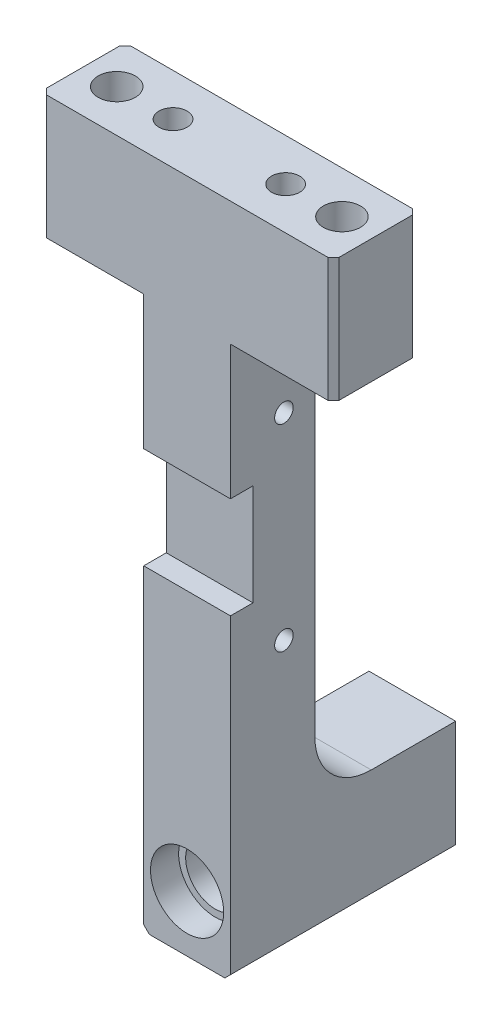
from build123d import *

# Parameters (mm, degrees)
SKETCH1_W                     = 52
SKETCH1_H                     = 120
BOSS_EXTRUDE1_DEPTH           = 7.5
SKETCH8_W                     = 18.3
SKETCH8_H                     = 98
CUT_EXTRUDE4_DEPTH            = 68.089492471
F_6_6_6_6_DIAMETER_HOLE1_D    = 6.6
CHAMFER1_SIZE                 = 1
BLIND_PIN_HOLE1_SIZE_MM_D     = 5
BLIND_PIN_HOLE1_SIZE_MM_DEPTH = 11
BLIND_PIN_HOLE1_SIZE_MM_TIP   = 1.502151548
BOSS_EXTRUDE2_DEPTH           = 25
FILLET1_R                     = 10
SKETCH14_R                    = 5.25
CUT_EXTRUDE5_DEPTH            = 77.655071587
SKETCH15_R                    = 6.5
CUT_EXTRUDE6_DEPTH            = 5
CUT_EXTRUDE7_START            = -5
SKETCH16_R                    = 6.5
CUT_EXTRUDE7_DEPTH            = 5
SKETCH17_W                    = 4
SKETCH17_H                    = 18
CUT_EXTRUDE8_DEPTH            = 77.104796169
M4_TAPPED_HOLE1_D             = 3.3
M4_TAPPED_HOLE1_DEPTH         = 10.1
M4_TAPPED_HOLE1_TIP           = 0.991420021


with BuildPart() as part:
    # Sketch1 → Boss-Extrude1 (new, symmetric)
    with BuildSketch(Plane.XY):
        Rectangle(SKETCH1_W, SKETCH1_H)
    extrude(amount=BOSS_EXTRUDE1_DEPTH, both=True)

    # Sketch8 → Cut-Extrude4 (cut, through all)
    with BuildSketch(Plane.XY.offset(7.5)):
        with Locations((-16.85, -11)):
            Rectangle(SKETCH8_W, SKETCH8_H)
    cut_extrude4 = extrude(amount=-CUT_EXTRUDE4_DEPTH, mode=Mode.SUBTRACT)

    # Mirror1: Cut-Extrude4 across plane
    add(cut_extrude4.mirror(Plane(origin=(0, 0, 0), x_dir=(0, 0, 1), z_dir=(1, 0, 0))), mode=Mode.SUBTRACT)

    # Ø6.6 (6.6) Diameter Hole1 (through all)
    with Locations(Plane(origin=(0, 60, 0), x_dir=(1, 0, 0), z_dir=(0, 1, 0))):
        with Locations((-20, 0), (20, 0)):
            Hole(F_6_6_6_6_DIAMETER_HOLE1_D / 2)

    # Chamfer1
    chamfer1_edges = [part.edges().sort_by_distance(p)[0] for p in [
        (-26, 49, 7.5),
        (-7.7, -60, 0),
        (26, 49, -7.5),
        (26, 49, 7.5),
        (7.7, -60, 0),
        (-26, 49, -7.5),
    ]]
    chamfer(chamfer1_edges, length=CHAMFER1_SIZE)

    # Blind Pin Hole1 size mm
    with Locations(Plane(origin=(0, 60, 0), x_dir=(1, 0, 0), z_dir=(0, 1, 0))):
        with Locations((-10, 0), (10, 0)):
            Hole(BLIND_PIN_HOLE1_SIZE_MM_D / 2, depth=BLIND_PIN_HOLE1_SIZE_MM_DEPTH)
            with Locations((0, 0, -(BLIND_PIN_HOLE1_SIZE_MM_DEPTH + BLIND_PIN_HOLE1_SIZE_MM_TIP / 2))):  # 118° drill point
                Cone(0, BLIND_PIN_HOLE1_SIZE_MM_D / 2, BLIND_PIN_HOLE1_SIZE_MM_TIP, mode=Mode.SUBTRACT)

    # Sketch13 → Boss-Extrude2 (add)
    with BuildSketch(Plane(origin=(0, 0, -7.5), x_dir=(-1, 0, 0), z_dir=(0, 0, -1))):
        Polygon((-7.7, -40), (7.7, -40), (7.7, -59), (6.7, -60), (-6.7, -60), (-7.7, -59), align=None)
    extrude(amount=BOSS_EXTRUDE2_DEPTH)

    # Fillet1
    fillet1_edges = [part.edges().sort_by_distance(p)[0] for p in [
        (0, -40, -7.5),
    ]]
    fillet(fillet1_edges, radius=FILLET1_R)

    # Sketch14 → Cut-Extrude5 (cut, through all)
    with BuildSketch(Plane.XY.offset(7.5)):
        with Locations((0, -50)):
            Circle(SKETCH14_R)
    extrude(amount=-CUT_EXTRUDE5_DEPTH, mode=Mode.SUBTRACT)

    # Sketch15 → Cut-Extrude6 (cut)
    with BuildSketch(Plane.XY.offset(7.5)):
        with Locations((0, -50)):
            Circle(SKETCH15_R)
    extrude(amount=-CUT_EXTRUDE6_DEPTH, mode=Mode.SUBTRACT)

    # Sketch16 → Cut-Extrude7 (cut)
    with BuildSketch(Plane(origin=(0, 0, -32.5), x_dir=(-1, 0, 0), z_dir=(0, 0, -1)).offset(CUT_EXTRUDE7_START)):
        with Locations(Location((0, -50, 0), (0, 0, 180))):
            Circle(SKETCH16_R)
    extrude(amount=CUT_EXTRUDE7_DEPTH, mode=Mode.SUBTRACT)

    # Sketch17 → Cut-Extrude8 (cut, through all)
    with BuildSketch(Plane(origin=(7.7, 0, 0), x_dir=(0, 0, -1), z_dir=(1, 0, 0))):
        with Locations((-5.5, 5.2)):
            Rectangle(SKETCH17_W, SKETCH17_H)
    extrude(amount=-CUT_EXTRUDE8_DEPTH, mode=Mode.SUBTRACT)

    # M4 Tapped Hole1
    with Locations(Plane(origin=(7.7, 0, 0), x_dir=(0, 0, -1), z_dir=(1, 0, 0))):
        with Locations((2, 22.7), (2, -12.3)):
            Hole(M4_TAPPED_HOLE1_D / 2, depth=M4_TAPPED_HOLE1_DEPTH)
            with Locations((0, 0, -(M4_TAPPED_HOLE1_DEPTH + M4_TAPPED_HOLE1_TIP / 2))):  # 118° drill point
                Cone(0, M4_TAPPED_HOLE1_D / 2, M4_TAPPED_HOLE1_TIP, mode=Mode.SUBTRACT)


solid = part.part
